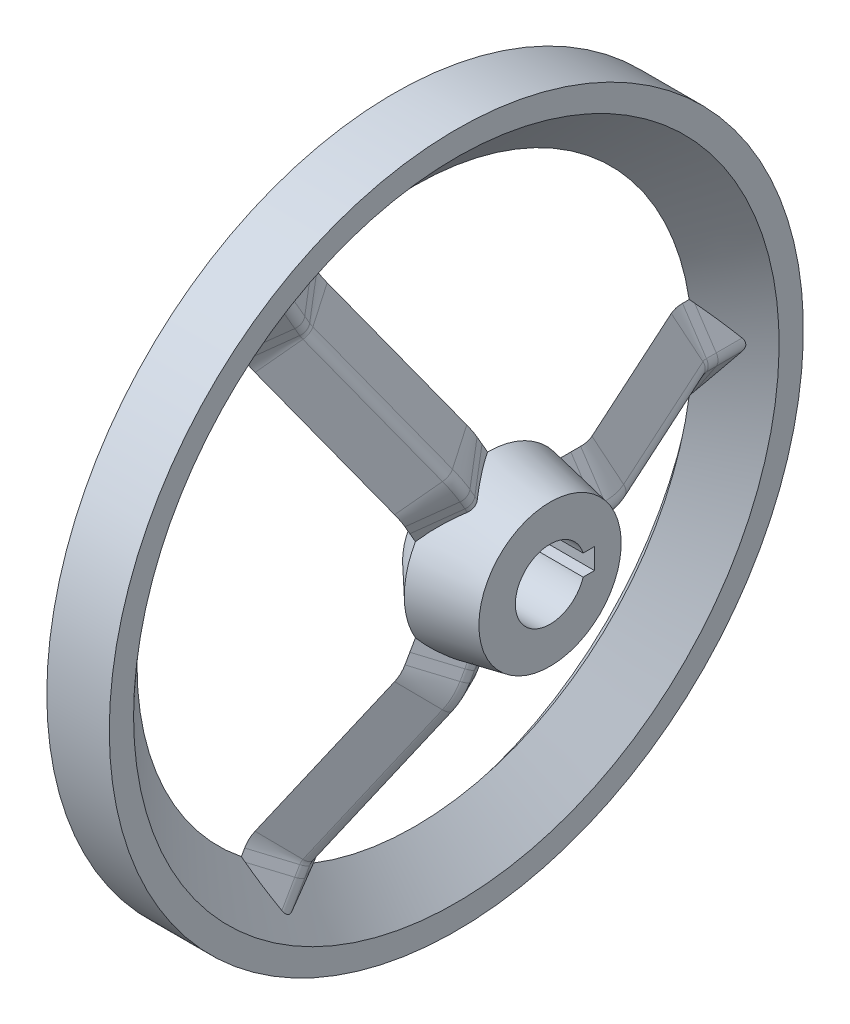
from build123d import *

# Parameters (mm, degrees)
PATTERN_CIRCULAR_1_COUNT = 3
EXTRUDE_1_REACH          = 148.7
SKETCH_4_R               = 13
SKETCH_5_W               = 5
SKETCH_5_H               = 6
CUT_EXTRUDE_1_DEPTH      = 147.700374941


with BuildPart() as part:
    # 草图1 → 旋转1 (revolve)
    with BuildSketch(Plane.XY, mode=Mode.PRIVATE) as revolve_1_sk:
        Polygon((0, 100), (0, 87.5), (6, 80), (18, 93), (18, 100), align=None)
        Polygon((27, 24), (45, 20.5), (45, 10), (18, 10), (18, 15.5), align=None)
    revolve(revolve_1_sk.sketch.rotate(Axis((0, 0, 0), (1, 0, 0)), 90), axis=Axis((0, 0, 0), (1, 0, 0)))

    # 扫描4: sweep along a path in 草图3
    with BuildLine(Plane(origin=(0, 0, 0), x_dir=(1, 0, 0), z_dir=(0, 1, 0))) as sweep_4_path:
        Line((27, 14), (27, 24))
        Line((27, 24), (27, 26.825339277))
        ThreePointArc((27, 26.825339277), (26.771611955, 28.950333349), (26.096880039, 30.978262773))
        Line((26.096880039, 30.978262773), (6.903119961, 73.021737227))
        ThreePointArc((6.903119961, 73.021737227), (6.228388045, 75.049666651), (6, 77.174660723))
        Line((6, 77.174660723), (6, 80))
        Line((6, 80), (6, 90))
    # 草图2 → 扫描4 (sweep)
    with BuildSketch(Plane.XY.offset(-14)):
        with BuildLine():
            Line((27, 12), (22.480769231, 1.153846154))
            ThreePointArc((22.480769231, 1.153846154), (22.25, 0), (22.480769231, -1.153846154))
            Line((22.480769231, -1.153846154), (27, -12))
            Line((27, -12), (33.890599608, -1.664100589))
            ThreePointArc((33.890599608, -1.664100589), (34.394448725, 0), (33.890599608, 1.664100589))
            Line((33.890599608, 1.664100589), (27, 12))
        make_face()
    sweep_4 = sweep(path=sweep_4_path.line)

    # 阵列(圆周)1: 扫描4 ×3 about axis
    pattern_circular_1_axis = Axis((0, 0, 0), (1, 0, 0))
    for i in range(1, PATTERN_CIRCULAR_1_COUNT):
        add(sweep_4.rotate(pattern_circular_1_axis, i * 360 / PATTERN_CIRCULAR_1_COUNT))

    # 凸台-拉伸1: up to this face of the body (flat: up to its plane)
    extrude_1_end = Plane(part.part.faces().sort_by_distance((0, 0, -97.171572875))[0])
    # 草图4 → 凸台-拉伸1 (add, up to the picked face)
    with BuildSketch(Plane.ZY.offset(-6), mode=Mode.PRIVATE) as extrude_1_sk1:
        with Locations((42.047439865, 72.828302174)):
            Circle(SKETCH_4_R)
    extrude_1_tool1 = split(extrude(extrude_1_sk1.sketch, amount=EXTRUDE_1_REACH, mode=Mode.PRIVATE), bisect_by=extrude_1_end, keep=Keep.BOTH, mode=Mode.PRIVATE)
    add(extrude_1_tool1.solids().sort_by(Axis((6, 72.828302, 42.04744), (-1, 0, 0)))[0])

    # 草图5 → 切除-拉伸1 (cut, through all)
    with BuildSketch(Plane.ZY.offset(-6)):
        with Locations((-10.3, 0)):
            Rectangle(SKETCH_5_W, SKETCH_5_H)
    extrude(amount=-CUT_EXTRUDE_1_DEPTH, mode=Mode.SUBTRACT)


solid = part.part
